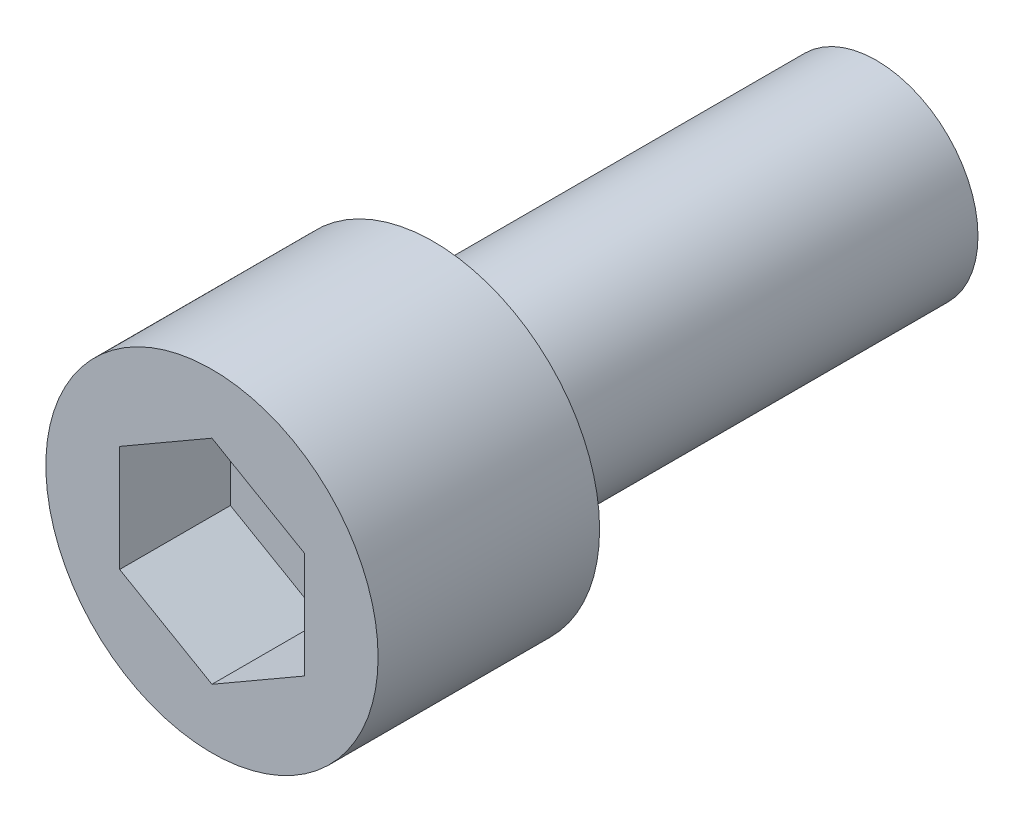
from build123d import *

# Parameters (mm, degrees)
SKETCH1_R           = 5.5
BOSS_EXTRUDE1_DEPTH = 24
SKETCH2_R           = 9
BOSS_EXTRUDE2_DEPTH = 12
CUT_EXTRUDE1_DEPTH  = 6


with BuildPart() as part:
    # Sketch1 → Boss-Extrude1 (new body)
    with BuildSketch(Plane.XY):
        Circle(SKETCH1_R)
    extrude(amount=BOSS_EXTRUDE1_DEPTH)

    # Sketch2 → Boss-Extrude2 (add)
    with BuildSketch(Plane.XY.offset(24)):
        Circle(SKETCH2_R)
    extrude(amount=BOSS_EXTRUDE2_DEPTH)

    # Sketch3 → Cut-Extrude1 (cut)
    with BuildSketch(Plane.XY.offset(36)):
        Polygon((0, 5.773502692), (-5, 2.886751346), (-5, -2.886751346), (0, -5.773502692), (5, -2.886751346), (5, 2.886751346), align=None)
    extrude(amount=-CUT_EXTRUDE1_DEPTH, mode=Mode.SUBTRACT)


solid = part.part
